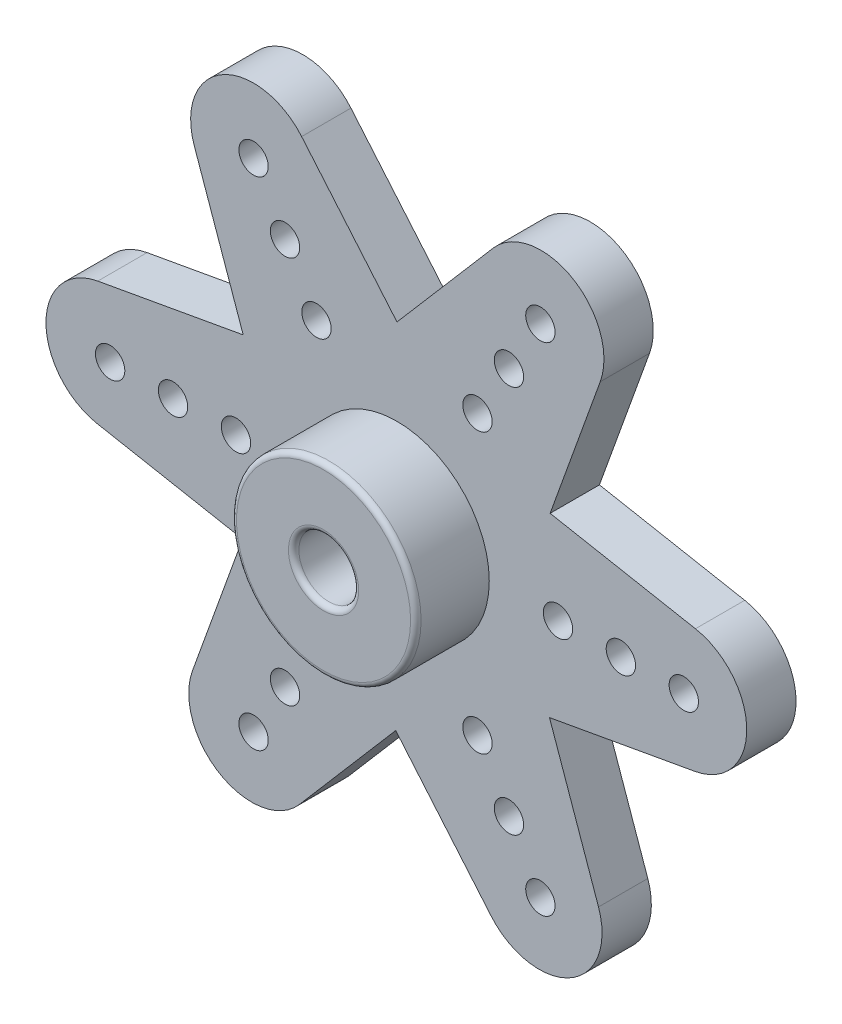
from build123d import *

# Parameters (mm, degrees)
SKETCH_1_R          = 0.7
EXTRUDE_1_DEPTH     = 2.35
SKETCH_2_R          = 4.4
EXTRUDE_2_DEPTH     = 3.5
SKETCH_3_R          = 1.425
CUT_EXTRUDE_1_DEPTH = 24.187779754
FILLET_1_R          = 0.25
SKETCH_4_R          = 4.25
SKETCH_4_R_2        = 3.5
CUT_EXTRUDE_2_DEPTH = 1
SKETCH_5_R          = 3
CUT_EXTRUDE_3_DEPTH = 1


with BuildPart() as part:
    # 草图1 → 凸台-拉伸1 (new body)
    with BuildSketch(Plane.XY):
        with BuildLine():
            Line((-4.545048295, 13.882270629), (0, 8.5))
            Line((0, 8.5), (4.591289657, 13.848716116))
            ThreePointArc((4.591289657, 13.848716116), (8.378143191, 14.486697202), (9.689930988, 10.877473971))
            Line((9.689930988, 10.877473971), (7.301272041, 4.250211371))
            Line((7.301272041, 4.250211371), (14.229040903, 2.94839595))
            ThreePointArc((14.229040903, 2.94839595), (16.674975498, -0.012124868), (14.20519039, -2.952778039))
            Line((14.20519039, -2.952778039), (7.271483148, -4.19777001))
            Line((7.271483148, -4.19777001), (9.607962353, -10.848301547))
            ThreePointArc((9.607962353, -10.848301547), (8.267043414, -14.446803451), (4.48547051, -13.778233392))
            Line((4.48547051, -13.778233392), (-0.059577785, -8.395962763))
            Line((-0.059577785, -8.395962763), (-4.650867443, -13.744678878))
            ThreePointArc((-4.650867443, -13.744678878), (-8.437720976, -14.382659965), (-9.749508773, -10.773436734))
            Line((-9.749508773, -10.773436734), (-7.360849826, -4.146174134))
            Line((-7.360849826, -4.146174134), (-14.288618688, -2.844358713))
            ThreePointArc((-14.288618688, -2.844358713), (-16.734553283, 0.116162105), (-14.264768176, 3.056815277))
            Line((-14.264768176, 3.056815277), (-7.331060933, 4.301807247))
            Line((-7.331060933, 4.301807247), (-9.667540138, 10.952338784))
            ThreePointArc((-9.667540138, 10.952338784), (-8.326621199, 14.550840688), (-4.545048295, 13.882270629))
        make_face()
        with Locations((13.675, 0)):
            Circle(SKETCH_1_R, mode=Mode.SUBTRACT)
        with Locations((10.675, 0)):
            Circle(SKETCH_1_R, mode=Mode.SUBTRACT)
        with Locations((7.675, 0)):
            Circle(SKETCH_1_R, mode=Mode.SUBTRACT)
        with Locations((3.8375, -6.646744974)):
            Circle(SKETCH_1_R, mode=Mode.SUBTRACT)
        with Locations((5.3375, -9.244821185)):
            Circle(SKETCH_1_R, mode=Mode.SUBTRACT)
        with Locations((6.8375, -11.842897397)):
            Circle(SKETCH_1_R, mode=Mode.SUBTRACT)
        with Locations((-3.8375, -6.646744974)):
            Circle(SKETCH_1_R, mode=Mode.SUBTRACT)
        with Locations((-5.3375, -9.244821185)):
            Circle(SKETCH_1_R, mode=Mode.SUBTRACT)
        with Locations((-6.8375, -11.842897397)):
            Circle(SKETCH_1_R, mode=Mode.SUBTRACT)
        with Locations((-7.675, 0)):
            Circle(SKETCH_1_R, mode=Mode.SUBTRACT)
        with Locations((-10.675, 0)):
            Circle(SKETCH_1_R, mode=Mode.SUBTRACT)
        with Locations((-13.675, 0)):
            Circle(SKETCH_1_R, mode=Mode.SUBTRACT)
        with Locations((-3.8375, 6.646744974)):
            Circle(SKETCH_1_R, mode=Mode.SUBTRACT)
        with Locations((-5.3375, 9.244821185)):
            Circle(SKETCH_1_R, mode=Mode.SUBTRACT)
        with Locations((-6.8375, 11.842897397)):
            Circle(SKETCH_1_R, mode=Mode.SUBTRACT)
        with Locations((3.8375, 6.646744974)):
            Circle(SKETCH_1_R, mode=Mode.SUBTRACT)
        with Locations((5.3375, 9.244821185)):
            Circle(SKETCH_1_R, mode=Mode.SUBTRACT)
        with Locations((6.8375, 11.842897397)):
            Circle(SKETCH_1_R, mode=Mode.SUBTRACT)
    extrude(amount=EXTRUDE_1_DEPTH)

    # 草图2 → 凸台-拉伸2 (add)
    with BuildSketch(Plane.XY.offset(2.35)):
        Circle(SKETCH_2_R)
    extrude(amount=EXTRUDE_2_DEPTH)

    # 草图3 → 切除-拉伸1 (cut, through all)
    with BuildSketch(Plane.XY.offset(5.85)):
        Circle(SKETCH_3_R)
    extrude(amount=-CUT_EXTRUDE_1_DEPTH, mode=Mode.SUBTRACT)

    # 圆角1
    fillet_1_edges = [part.edges().sort_by_distance(p)[0] for p in [
        (-4.4, 0, 5.85),
        (-1.425, 0, 5.85),
    ]]
    fillet(fillet_1_edges, radius=FILLET_1_R)

    # 草图4 → 切除-拉伸2 (cut)
    with BuildSketch(Plane(origin=(0, 0, 0), x_dir=(-1, 0, 0), z_dir=(0, 0, -1))):
        Circle(SKETCH_4_R)
        Circle(SKETCH_4_R_2, mode=Mode.SUBTRACT)
    extrude(amount=-CUT_EXTRUDE_2_DEPTH, mode=Mode.SUBTRACT)

    # 草图5 → 切除-拉伸3 (cut)
    with BuildSketch(Plane(origin=(0, 0, 0), x_dir=(-1, 0, 0), z_dir=(0, 0, -1))):
        Circle(SKETCH_5_R)
    extrude(amount=-CUT_EXTRUDE_3_DEPTH, mode=Mode.SUBTRACT)


solid = part.part
